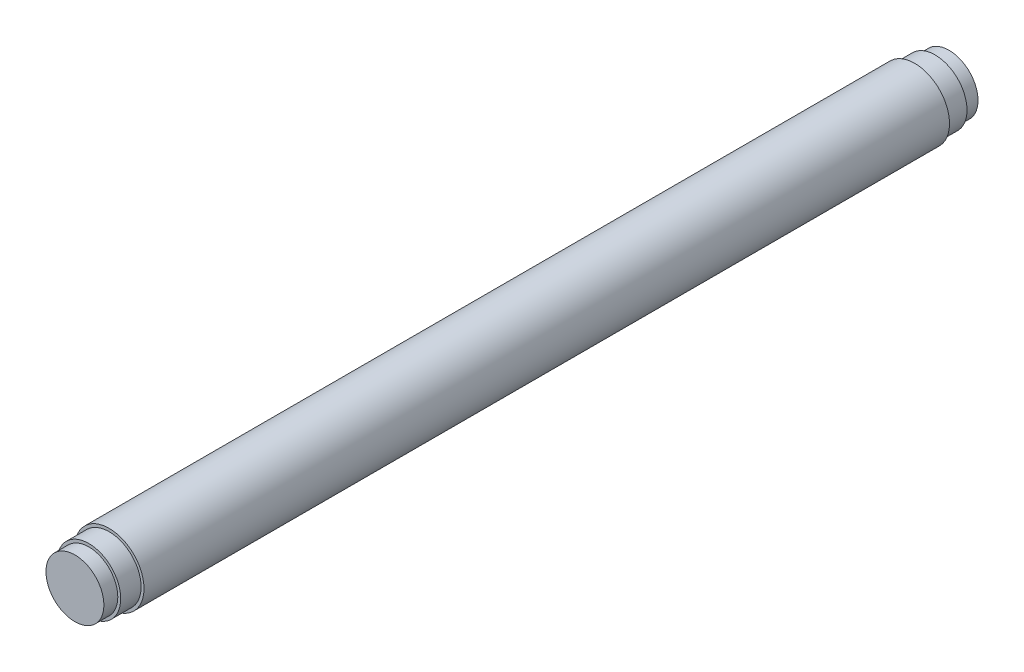
SolidWorks part; units mm, degrees
material "普通碳钢"
ref_plane "Front Plane" through (0, 0, 0) normal (0, 0, 1) x (1, 0, 0)
ref_plane "Top Plane" through (0, 0, 0) normal (0, 1, 0) x (1, 0, 0)
ref_plane "Right Plane" through (0, 0, 0) normal (1, 0, 0) x (0, 0, -1)
sketch "Sketch1" plane through (0, 0, 0) normal (0, 0, 1) x (1, 0, 0)
  circle A0 centre (0, 0) radius 27.5
  dimension "D1" = 55
extrude "Boss-Extrude1" add sketch "Sketch1" along normal blind 17.6
sketch "Sketch2" plane through (0, 0, 0) normal (0, 0, -1) x (-1, 0, 0)
  circle A0 centre (0, 0) radius 25
  dimension "D1" = 50
extrude "Boss-Extrude2" add sketch "Sketch2" along normal blind 12
sketch "Sketch3" plane through (0, 0, 17.6) normal (0, 0, 1) x (1, 0, 0)
  circle A0 centre (0, 0) radius 30
  dimension "D1" = 60
extrude "Boss-Extrude3" add sketch "Sketch3" along normal blind 695
sketch "Sketch4" plane through (0, 0, 712.6) normal (0, 0, 1) x (1, 0, 0)
  circle A0 centre (0, 0) radius 27.5
  dimension "D1" = 55
extrude "Boss-Extrude4" add sketch "Sketch4" along normal blind 17.6
sketch "Sketch5" plane through (0, 0, 730.2) normal (0, 0, 1) x (1, 0, 0)
  circle A0 centre (0, 0) radius 25
  dimension "D1" = 50
extrude "Boss-Extrude5" add sketch "Sketch5" along normal blind 12
